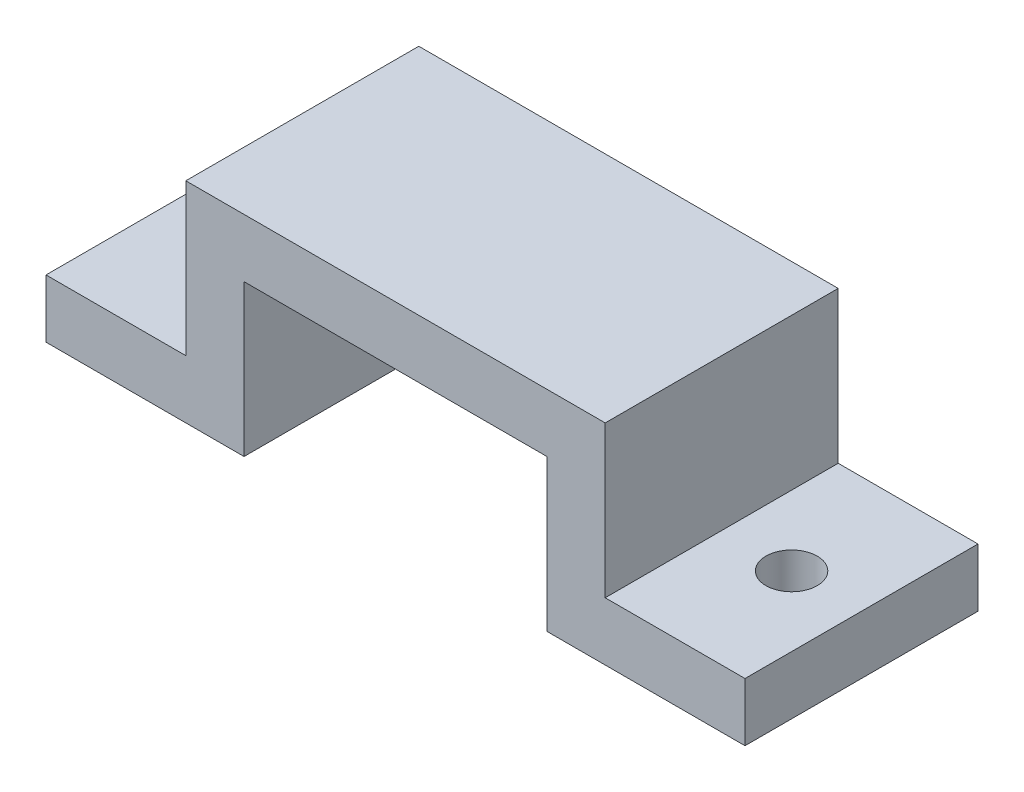
SolidWorks part; units mm, degrees
ref_plane "前视基准面" through (0, 0, 0) normal (0, 0, 1) x (1, 0, 0)
ref_plane "上视基准面" through (0, 0, 0) normal (0, 1, 0) x (1, 0, 0)
ref_plane "右视基准面" through (0, 0, 0) normal (1, 0, 0) x (0, 0, -1)
sketch "草图1" plane through (0, 0, 0) normal (0, 0, 1) x (1, 0, 0)
  line L0 (0, 0) -> (17, 0)
  line L5 (17, 0) -> (17, 13)
  line L6 (17, 13) -> (43, 13)
  line L11 (43, 13) -> (43, 0)
  line L12 (43, 0) -> (60, 0)
  line L13 (60, 0) -> (60, 5)
  line L14 (60, 5) -> (48, 5)
  line L15 (48, 5) -> (48, 18)
  line L16 (48, 18) -> (12, 18)
  line L17 (12, 18) -> (12, 5)
  line L18 (12, 5) -> (0, 5)
  line L19 (0, 5) -> (0, 0)
  line L20 (17, 18) -> (17, 13) construction
  line L21 (48, 5) -> (43, 5) construction
  line L22 (17, 13) -> (12, 13) construction
  dimension "D1" = 5
  dimension "D2" = 26
  dimension "D3" = 13
  dimension "D4" = 12
extrude "凸台-拉伸1" add sketch "草图1" along normal mid plane 20
sketch "草图2" plane through (0, 5, 0) normal (0, 1, 0) x (1, 0, 0)
  line L0 (0, 0) -> (12, 0) construction
  line L1 (0, -10) -> (0, 10) construction
  line L2 (12, 0) -> (48, 0) construction
  line L3 (48, -10) -> (48, 10) construction
  line L4 (48, 0) -> (60, 0) construction
  line L5 (60, -10) -> (60, 10) construction
  line L6 (12, -10) -> (12, 10) construction
  circle A0 centre (6, 0) radius 2.2
  circle A1 centre (54, 0) radius 2.2
  dimension "D1" = 4.4
extrude "切除-拉伸1" cut sketch "草图2" against normal blind 10
